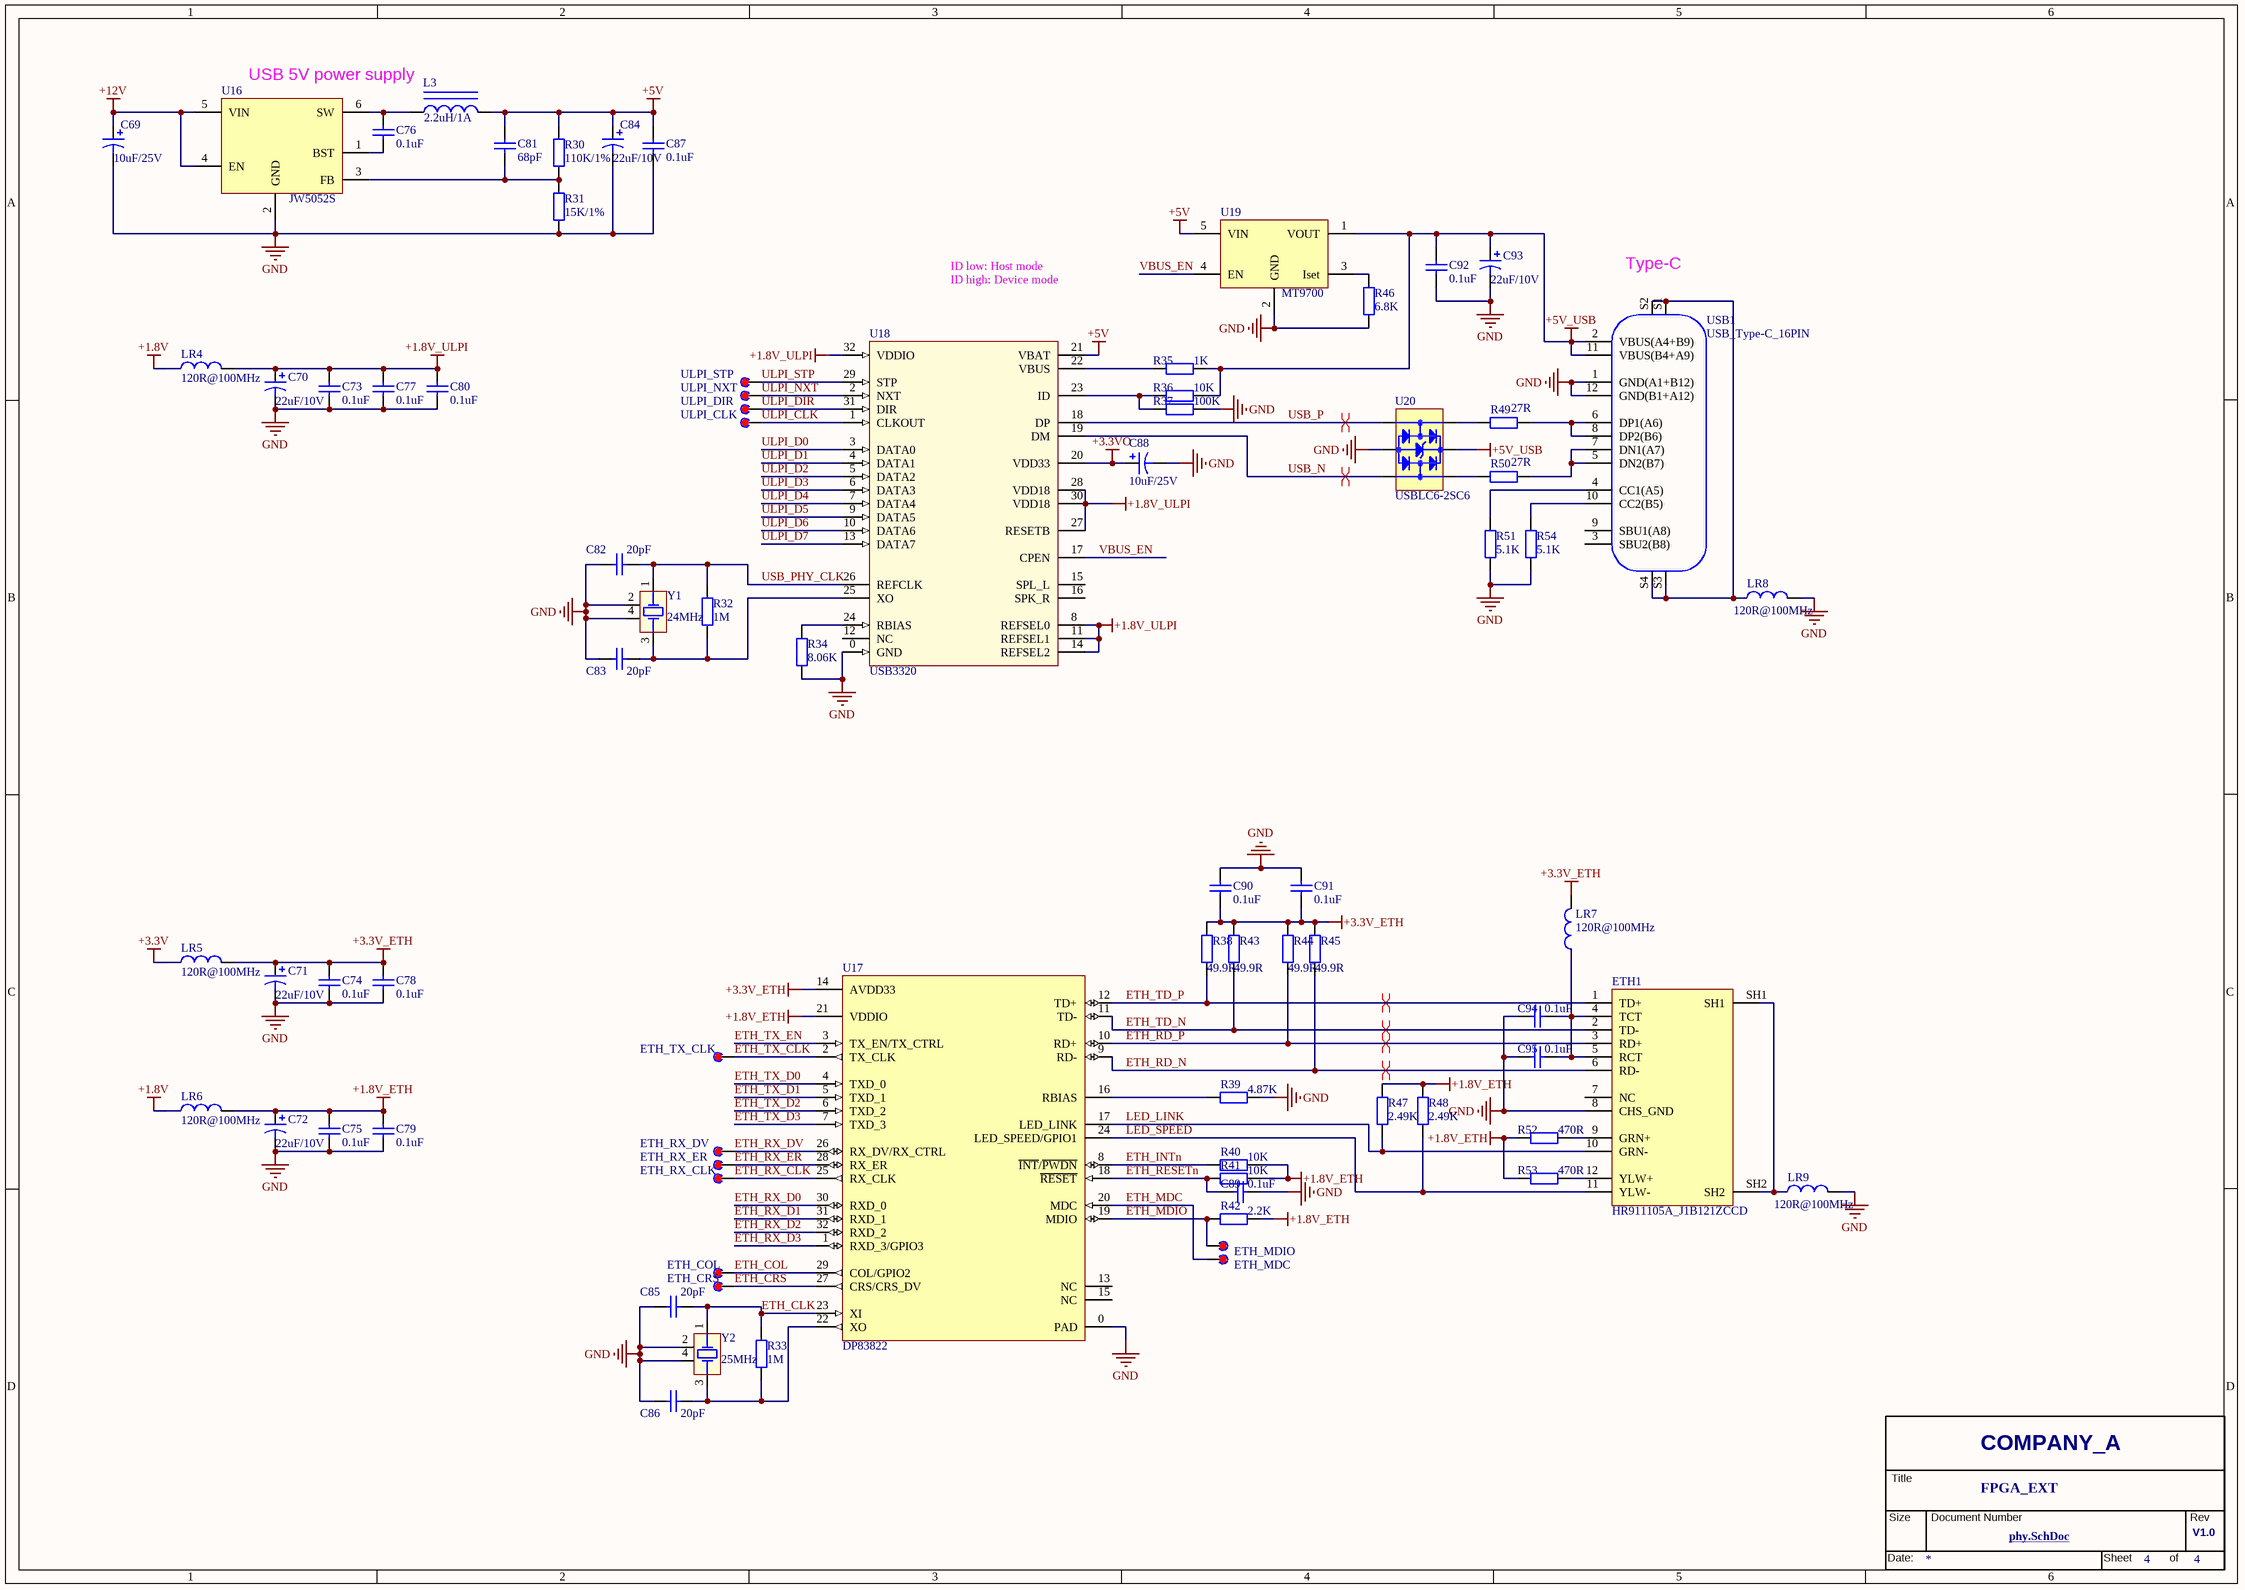
[diagram p0: MISC105414-8.SchDoc]
# Altium project MISC105414-4.PrjPcb (part 3 of 3)

## Sheet MISC105414-8.SchDoc
size 420 x 297 mm; DocumentNumber: MISC105414; SheetNumber: 4; SheetTotal: 4

### Parts
(Parts that share a designator on the sheet are numbered #1, #2 ... from top to bottom, then left to right.)
*?#4  Page Count: 4  OrgName: COMPANY_A  Title: FPGA_EXT  RevCode: V1.0  Doc: phy.SchDoc  (hidden comment: TitleBlock_YHSCH)  (graphical)
C69  10uF/25V  [0603C_N]
C70  22uF/10V  [0603C_N]
C71  22uF/10V  [0603C_N]
C72  22uF/10V  [0603C_N]
C73  0.1uF  [0603C_N]
C74  0.1uF  [0603C_N]
C75  0.1uF  [0603C_N]
C76  0.1uF  [0603C_N]
C77  0.1uF  [0603C_N]
C78  0.1uF  [0603C_N]
C79  0.1uF  [0603C_N]
C80  0.1uF  [0603C_N]
C81  68pF  [0603C_N]
C82  20pF  [0603C_N]
C83  20pF  [0603C_N]
C84  22uF/10V  [0603C_N]
C85  20pF  [0603C_N]
C86  20pF  [0603C_N]
C87  0.1uF  [0603C_N]
C88  10uF/25V  [0603C_N]
C89  0.1uF  [0603C_N]
C90  0.1uF  [0603C_N]
C91  0.1uF  [0603C_N]
C92  0.1uF  [0603C_N]
C93  22uF/10V  [0603C_N]
C94  0.1uF  [0603C_N]
C95  0.1uF  [0603C_N]
ETH1  HR911105A_J1B121ZCCD  [RJ45_HR911003A]
L3  2.2uH/1A  [LD-5.5mm]
LR4  120R@100MHz  [0603R_N]
LR5  120R@100MHz  [0603R_N]
LR6  120R@100MHz  [0603R_N]
LR7  120R@100MHz  [0603R_N]
LR8  120R@100MHz  [0603R_N]
LR9  120R@100MHz  [0603R_N]
R30  110K/1%  [0603R_N]
R31  15K/1%  [0603R_N]
R32  1M  [0603R_N]
R33  1M  [0603R_N]
R34  8.06K  [0603R_N]
R35  1K  [0603R_N]
R36  10K  [0603R_N]
R37  100K  [0603R_N]
R38  49.9R  [0603R_N]
R39  4.87K  [0603R_N]
R40  10K  [0603R_N]
R41  10K  [0603R_N]
R42  2.2K  [0603R_N]
R43  49.9R  [0603R_N]
R44  49.9R  [0603R_N]
R45  49.9R  [0603R_N]
R46  6.8K  [0603R_N]
R47  2.49K  [0603R_N]
R48  2.49K  [0603R_N]
R49  27R  [0603R_N]
R50  27R  [0603R_N]
R51  5.1K  [0603R_N]
R52  470R  [0603R_N]
R53  470R  [0603R_N]
R54  5.1K  [0603R_N]
TP40  ETH_TX_CLK  [FZ_TP-SMD-Mini]
TP41  ETH_RX_DV  [FZ_TP-SMD-Mini]
TP42  ETH_RX_ER  [FZ_TP-SMD-Mini]
TP43  ETH_RX_CLK  [FZ_TP-SMD-Mini]
TP44  ETH_COL  [FZ_TP-SMD-Mini]
TP45  ETH_CRS  [FZ_TP-SMD-Mini]
TP46  ULPI_STP  [FZ_TP-SMD-Mini]
TP47  ULPI_NXT  [FZ_TP-SMD-Mini]
TP48  ULPI_DIR  [FZ_TP-SMD-Mini]
TP49  ULPI_CLK  [FZ_TP-SMD-Mini]
TP50  ETH_MDIO  [FZ_TP-SMD-Mini]
TP51  ETH_MDC  [FZ_TP-SMD-Mini]
U16  JW5052S  [SOT-23-6]
U17  DP83822  [QFN32 5X5]
U18  USB3320  [QFN32 5x5]
U19  MT9700  [SOT-23-5]
U20  USBLC6-2SC6  [SOT-23-6]
USB1  USB_Type-C_16PIN  [USB_Type-C_16PIN]
Y1  24MHz  [XTAL_SMD3225]
Y2  25MHz  [XTAL_SMD3225]

### Nets
+1.8V: LR4.2 LR6.2
+1.8V_ETH: C72.1 C75.2 C79.2 LR6.1 R40.1 R41.1 R42.1 R47.1 R48.1 R52.1 R53.1 U17.21(VDDIO)
+1.8V_ULPI: C70.1 C73.2 C77.2 C80.1 LR4.1 U18.8(REFSEL0) U18.11(REFSEL1) U18.14(REFSEL2) U18.27(RESETB) U18.28(VDD18) U18.30(VDD18) U18.32(VDDIO)
+3.3V: LR5.2
+3.3V_ETH: C71.1 C74.2 C78.2 C90.2 C91.2 LR5.1 LR7.1 R38.2 R43.2 R44.2 R45.2 U17.14(AVDD33)
+3.3VO: C88.1 U18.20(VDD33)
+5V: C81.1 C84.1 C87.2 L3.2 R30.1 U18.21(VBAT) U19.5(VIN)
+5V_USB: C92.1 C93.1 R35.2 R36.2 U19.1(VOUT) U20.5(Vbus) USB1.2(VBUS(A4+B9)) USB1.11(VBUS(B4+A9))
+12V: C69.1 U16.4(EN) U16.5(VIN)
GND: C69.2 C70.2 C71.2 C72.2 C73.1 C74.1 C75.1 C77.1 C78.1 C79.1 C80.2 C82.2 C83.2 C84.2 C85.2 C86.2 C87.1 C88.2 C89.1 C90.1 C91.1 C92.2 C93.2 C94.1 C95.1 ETH1.8(CHS_GND) LR8.1 LR9.1 R31.2 R34.2 R37.2 R39.1 R46.1 R51.1 R54.1 U16.2(GND) U17.0(PAD) U18.0(GND) U19.2(GND) U20.2(GND) USB1.1(GND(A1+B12)) USB1.12(GND(B1+A12)) Y1.2 Y1.4 Y2.2 Y2.4
ETH_CLK: C85.1 R33.2 U17.23(XI) Y2.1(OSC1)
ETH_COL: TP44.1 U17.29(COL/GPIO2)
ETH_CRS: TP45.1 U17.27(CRS/CRS_DV)
ETH_INTn: R40.2 U17.8(~{INT}/~{PWDN})
ETH_MDC: TP51.1 U17.20(MDC)
ETH_MDIO: R42.2 TP50.1 U17.19(MDIO)
ETH_RD_N: ETH1.6(RD-) R45.1 U17.9(RD-)
ETH_RD_P: ETH1.3(RD+) R44.1 U17.10(RD+)
ETH_RESETn: C89.2 R41.2 U17.18(~{RESET})
ETH_RX_CLK: TP43.1 U17.25(RX_CLK)
ETH_RX_D0: U17.30(RXD_0)
ETH_RX_D1: U17.31(RXD_1)
ETH_RX_D2: U17.32(RXD_2)
ETH_RX_D3: U17.1(RXD_3/GPIO3)
ETH_RX_DV: TP41.1 U17.26(RX_DV/RX_CTRL)
ETH_RX_ER: TP42.1 U17.28(RX_ER)
ETH_TD_N: ETH1.2(TD-) R43.1 U17.11(TD-)
ETH_TD_P: ETH1.1(TD+) R38.1 U17.12(TD+)
ETH_TX_CLK: TP40.1 U17.2(TX_CLK)
ETH_TX_D0: U17.4(TXD_0)
ETH_TX_D1: U17.5(TXD_1)
ETH_TX_D2: U17.6(TXD_2)
ETH_TX_D3: U17.7(TXD_3)
ETH_TX_EN: U17.3(TX_EN/TX_CTRL)
LED_LINK: ETH1.10(GRN-) R47.2 U17.17(LED_LINK)
LED_SPEED: ETH1.11(YLW-) R48.2 U17.24(LED_SPEED/GPIO1)
ULPI_CLK: TP49.1 U18.1(CLKOUT)
ULPI_D0: U18.3(DATA0)
ULPI_D1: U18.4(DATA1)
ULPI_D2: U18.5(DATA2)
ULPI_D3: U18.6(DATA3)
ULPI_D4: U18.7(DATA4)
ULPI_D5: U18.9(DATA5)
ULPI_D6: U18.10(DATA6)
ULPI_D7: U18.13(DATA7)
ULPI_DIR: TP48.1 U18.31(DIR)
ULPI_NXT: TP47.1 U18.2(NXT)
ULPI_STP: TP46.1 U18.29(STP)
USB_N: U18.19(DM) U20.1(CH1)
USB_P: U18.18(DP) U20.3(CH2)
USB_PHY_CLK: C82.1 R32.2 U18.26(REFCLK) Y1.1(OSC1)
VBUS_EN: U18.17(CPEN) U19.4(EN)
NetC76_1: C76.1 U16.1(BST)
NetC76_2: C76.2 L3.1 U16.6(SW)
NetC81_2: C81.2 R30.2 R31.1 U16.3(FB)
NetC83_1: C83.1 R32.1 U18.25(XO) Y1.3(OSC2)
NetC86_1: C86.1 R33.1 U17.22(XO) Y2.3(OSC2)
NetC94_2: C94.2 C95.2 ETH1.4(TCT) ETH1.5(RCT) LR7.2
NetETH1_9: ETH1.9(GRN+) R52.2
NetETH1_12: ETH1.12(YLW+) R53.2
NetETH1_SH1: ETH1.SH1 ETH1.SH2 LR9.2
NetLR8_2: LR8.2 USB1.S1 USB1.S2 USB1.S3 USB1.S4
NetR34_1: R34.1 U18.24(RBIAS)
NetR35_1: R35.1 U18.22(VBUS)
NetR36_1: R36.1 R37.1 U18.23(ID)
NetR39_2: R39.2 U17.16(RBIAS)
NetR46_2: R46.2 U19.3(Iset)
NetR49_1: R49.1 U20.4(CH3)
NetR49_2: R49.2 USB1.6(DP1(A6)) USB1.8(DP2(B6))
NetR50_1: R50.1 U20.6(CH4)
NetR50_2: R50.2 USB1.5(DN2(B7)) USB1.7(DN1(A7))
NetR51_2: R51.2 USB1.4(CC1(A5))
NetR54_2: R54.2 USB1.10(CC2(B5))

Not connected (* = marked no-connect by the designer): ETH1 7(NC); U17 13(NC) 15(NC); U18 12(NC) 15(SPL_L) 16(SPK_R); USB1 3(SBU2(B8)) 9(SBU1(A8))

### Layout directives
differential pair: ETH_RD_N, ETH_RD_P, ETH_TD_N, ETH_TD_P, USB_N, USB_P

### Notes on the sheet
- USB 5V power supply
- ID low: Host mode
- ID high: Device mode
- (near USB1) Type-C

### Library data of the parts
*?#4 = TitleBlock_YHSCH: Cage Code: 1; Page Number: 4; Page Modify Date: *
C69-C72 C84 C88 C93 = Cap Pol1: Polarized Capacitor (Radial); Value: 1uF; Published: 8-Jun-2000; LatestRevisionDate: 17-Jul-2002; LatestRevisionNote: Re-released for DXP Platform.; PackageReference: RB7.6-15; Publisher: Altium Limited
C73-C81 C87 C89-C92 C94 C95 = Cap: Capacitor; Value: 100nF; Published: 8-Jun-2000; LatestRevisionDate: 17-Jul-2002; LatestRevisionNote: Re-released for DXP Platform.; PackageReference: RAD-0.3; Publisher: Altium Limited
C82 C83 C85 C86 = Cap: Capacitor; Value: 0.1uF; Published: 8-Jun-2000; LatestRevisionDate: 17-Jul-2002; LatestRevisionNote: Re-released for DXP Platform.; PackageReference: RAD-0.3; Publisher: Altium Limited
ETH1 = HR911105A
L3 = Inductor Iron: Magnetic-Core Inductor; Published: 24-Mar-1999; LatestRevisionDate: 17-Jul-2002; LatestRevisionNote: Re-released for DXP Platform.; PackageReference: AXIAL-0.9; PackageDescription: Axial Device, Thru-Hole; 2 Leads; 0.9 in Pin Spacing; Publisher: Altium Limited
LR4-LR9 = L
R30-R54 = Res2: Resistor; Value: 4.7K; Published: 8-Jun-2000; LatestRevisionDate: 17-Jul-2002; LatestRevisionNote: Re-released for DXP Platform.; PackageReference: AXIAL-0.4; Publisher: Altium Limited
TP40-TP51 = TP_SMD
U16 = MP2359_JW5052S_SY8113B
U17 = DP83822_Eth PHY 10_100M w1588 802.3az
U18 = USB3320: USB_HS ULPI PHY
U19 = LPW5209_MT9700: Power switch 3.3V/5V
Y1 Y2 = XTAL_2

## Nets that join several sheets
+1.8V: MISC105414-3 (J1.E39 J1.F40 J1.G39 J1.H40), MISC105414-2 (5 pins), MISC105414-7 (45 pins), MISC105414-8 (LR4.2 LR6.2)
+3.3V: MISC105414-3 (5 pins), MISC105414-2 (13 pins), MISC105414-8 (LR5.2)
+12V: MISC105414-3 (5 pins), MISC105414-8 (C69.1 U16.4 U16.5)
GND: MISC105414-3 (244 pins), MISC105414-2 (70 pins), MISC105414-7 (45 pins), MISC105414-8 (46 pins)
DVP_D0: MISC105414-3 (J1.F16), MISC105414-2 (J5.24 R24.2)
DVP_D1: MISC105414-3 (J1.E16), MISC105414-2 (J5.23 R23.2)
DVP_D2: MISC105414-3 (J1.E13), MISC105414-2 (J5.19)
DVP_D3: MISC105414-3 (J1.F14), MISC105414-2 (J5.21)
DVP_D4: MISC105414-3 (J1.E15), MISC105414-2 (J5.22)
DVP_D5: MISC105414-3 (J1.F13), MISC105414-2 (J5.20)
DVP_D6: MISC105414-3 (J1.E12), MISC105414-2 (J5.18)
DVP_D7: MISC105414-3 (J1.F10), MISC105414-2 (J5.16)
DVP_D8: MISC105414-3 (J1.E10), MISC105414-2 (J5.14)
DVP_D9: MISC105414-3 (J1.E9), MISC105414-2 (J5.12)
DVP_HSYNC: MISC105414-3 (J1.E7), MISC105414-2 (J5.9 TP12.1)
DVP_MCLK: MISC105414-3 (J1.F8), MISC105414-2 (J5.13 TP16.1)
DVP_PCLK: MISC105414-3 (J1.F11), MISC105414-2 (J5.17 TP17.1)
DVP_PWDN: MISC105414-3 (J1.F7), MISC105414-2 (J5.8 TP11.1)
DVP_RST: MISC105414-3 (J1.E3), MISC105414-2 (J5.6 TP15.1)
DVP_SCL: MISC105414-3 (J1.F5), MISC105414-2 (J5.5 R26.1 TP14.1)
DVP_SDA: MISC105414-3 (J1.F4), MISC105414-2 (J5.3 R27.1 TP13.1)
DVP_STROBE: MISC105414-3 (J1.E2), MISC105414-2 (J5.1)
DVP_VSYNC: MISC105414-3 (J1.E6), MISC105414-2 (J5.7 TP10.1)
ETH_CLK: MISC105414-3 (J1.A38), MISC105414-8 (C85.1 R33.2 U17.23 Y2.1)
ETH_COL: MISC105414-3 (J1.K38), MISC105414-8 (TP44.1 U17.29)
ETH_CRS: MISC105414-3 (J1.G37), MISC105414-8 (TP45.1 U17.27)
ETH_INTn: MISC105414-3 (J1.K31), MISC105414-8 (R40.2 U17.8)
ETH_MDC: MISC105414-3 (J1.H31), MISC105414-8 (TP51.1 U17.20)
ETH_MDIO: MISC105414-3 (J1.H32), MISC105414-8 (R42.2 TP50.1 U17.19)
ETH_RESETn: MISC105414-3 (J1.K32), MISC105414-8 (C89.2 R41.2 U17.18)
ETH_RX_CLK: MISC105414-3 (J1.H38), MISC105414-8 (TP43.1 U17.25)
ETH_RX_D0: MISC105414-3 (J1.J37), MISC105414-8 (U17.30)
ETH_RX_D1: MISC105414-3 (J1.J36), MISC105414-8 (U17.31)
ETH_RX_D2: MISC105414-3 (J1.H35), MISC105414-8 (U17.32)
ETH_RX_D3: MISC105414-3 (J1.H34), MISC105414-8 (U17.1)
ETH_RX_DV: MISC105414-3 (J1.H37), MISC105414-8 (TP41.1 U17.26)
ETH_RX_ER: MISC105414-3 (J1.G36), MISC105414-8 (TP42.1 U17.28)
ETH_TX_CLK: MISC105414-3 (J1.G34), MISC105414-8 (TP40.1 U17.2)
ETH_TX_D0: MISC105414-3 (J1.K35), MISC105414-8 (U17.4)
ETH_TX_D1: MISC105414-3 (J1.K34), MISC105414-8 (U17.5)
ETH_TX_D2: MISC105414-3 (J1.J34), MISC105414-8 (U17.6)
ETH_TX_D3: MISC105414-3 (J1.J33), MISC105414-8 (U17.7)
ETH_TX_EN: MISC105414-3 (J1.G33), MISC105414-8 (U17.3)
EXT_IO0: MISC105414-3 (J1.Y2), MISC105414-2 (JE1.3)
EXT_IO1: MISC105414-3 (J1.A2), MISC105414-2 (JE1.4)
EXT_IO2: MISC105414-3 (J1.Y3), MISC105414-2 (JE1.5)
EXT_IO3: MISC105414-3 (J1.A3), MISC105414-2 (JE1.6)
EXT_IO4: MISC105414-3 (J1.Z4), MISC105414-2 (JE1.7)
EXT_IO5: MISC105414-3 (J1.B4), MISC105414-2 (JE1.8)
EXT_IO6: MISC105414-3 (J1.Z5), MISC105414-2 (JE1.9)
EXT_IO7: MISC105414-3 (J1.B5), MISC105414-2 (JE1.10)
EXT_IO8: MISC105414-3 (J1.Y6), MISC105414-2 (JE1.11)
EXT_IO9: MISC105414-3 (J1.A6), MISC105414-2 (JE1.12)
EXT_IO10: MISC105414-3 (J1.Y7), MISC105414-2 (JE1.13)
EXT_IO11: MISC105414-3 (J1.A7), MISC105414-2 (JE1.14)
EXT_IO12: MISC105414-3 (J1.Z8), MISC105414-2 (JE1.15)
EXT_IO13: MISC105414-3 (J1.B8), MISC105414-2 (JE1.16)
EXT_IO14: MISC105414-3 (J1.Z9), MISC105414-2 (JE1.17)
EXT_IO15: MISC105414-3 (J1.B9), MISC105414-2 (JE1.18)
EXT_IO16: MISC105414-3 (J1.Y10), MISC105414-2 (JE1.23)
EXT_IO17: MISC105414-3 (J1.A10), MISC105414-2 (JE1.24)
EXT_IO18: MISC105414-3 (J1.Y11), MISC105414-2 (JE1.25)
EXT_IO19: MISC105414-3 (J1.A11), MISC105414-2 (JE1.26)
EXT_IO20: MISC105414-3 (J1.Z12), MISC105414-2 (JE1.27)
EXT_IO21: MISC105414-3 (J1.B12), MISC105414-2 (JE1.28)
EXT_IO22: MISC105414-3 (J1.Z13), MISC105414-2 (JE1.29)
EXT_IO23: MISC105414-3 (J1.B13), MISC105414-2 (JE1.30)
EXT_IO24: MISC105414-3 (J1.Y14), MISC105414-2 (JE1.31)
EXT_IO25: MISC105414-3 (J1.A14), MISC105414-2 (JE1.32)
EXT_IO26: MISC105414-3 (J1.Y15), MISC105414-2 (JE1.33)
EXT_IO27: MISC105414-3 (J1.A15), MISC105414-2 (JE1.34)
EXT_IO28: MISC105414-3 (J1.Z16), MISC105414-2 (JE1.35)
EXT_IO29: MISC105414-3 (J1.B16), MISC105414-2 (JE1.36)
EXT_IO30: MISC105414-3 (J1.Z17), MISC105414-2 (JE1.37)
EXT_IO31: MISC105414-3 (J1.B17), MISC105414-2 (JE1.38)
EXT_IO32: MISC105414-3 (J1.Y18), MISC105414-2 (JE2.3)
EXT_IO33: MISC105414-3 (J1.A18), MISC105414-2 (JE2.4)
EXT_IO34: MISC105414-3 (J1.Y19), MISC105414-2 (JE2.5)
EXT_IO35: MISC105414-3 (J1.A19), MISC105414-2 (JE2.6)
EXT_IO36: MISC105414-3 (J1.Z20), MISC105414-2 (JE2.7)
EXT_IO37: MISC105414-3 (J1.B20), MISC105414-2 (JE2.8)
EXT_IO38: MISC105414-3 (J1.Z21), MISC105414-2 (JE2.9)
EXT_IO39: MISC105414-3 (J1.B21), MISC105414-2 (JE2.10)
EXT_IO40: MISC105414-3 (J1.Y22), MISC105414-2 (JE2.11)
EXT_IO41: MISC105414-3 (J1.A22), MISC105414-2 (JE2.12)
EXT_IO42: MISC105414-3 (J1.Y23), MISC105414-2 (JE2.13)
EXT_IO43: MISC105414-3 (J1.A23), MISC105414-2 (JE2.14)
EXT_IO44: MISC105414-3 (J1.Z24), MISC105414-2 (JE2.15)
EXT_IO45: MISC105414-3 (J1.B24), MISC105414-2 (JE2.16)
EXT_IO46: MISC105414-3 (J1.Z25), MISC105414-2 (JE2.17)
EXT_IO47: MISC105414-3 (J1.B25), MISC105414-2 (JE2.18)
EXT_IO48: MISC105414-3 (J1.Y26), MISC105414-2 (JE2.23)
EXT_IO49: MISC105414-3 (J1.A26), MISC105414-2 (JE2.24)
EXT_IO50: MISC105414-3 (J1.Y27), MISC105414-2 (JE2.25)
EXT_IO51: MISC105414-3 (J1.A27), MISC105414-2 (JE2.26)
EXT_IO52: MISC105414-3 (J1.Z28), MISC105414-2 (JE2.27)
EXT_IO53: MISC105414-3 (J1.B28), MISC105414-2 (JE2.28)
EXT_IO54: MISC105414-3 (J1.Z29), MISC105414-2 (JE2.29)
EXT_IO55: MISC105414-3 (J1.B29), MISC105414-2 (JE2.30)
EXT_IO56: MISC105414-3 (J1.Y30), MISC105414-2 (JE2.31)
EXT_IO57: MISC105414-3 (J1.A30), MISC105414-2 (JE2.32)
EXT_IO58: MISC105414-3 (J1.Y31), MISC105414-2 (JE2.33)
EXT_IO59: MISC105414-3 (J1.A31), MISC105414-2 (JE2.34)
EXT_IO60: MISC105414-3 (J1.B32), MISC105414-2 (JE2.35)
EXT_IO61: MISC105414-3 (J1.B33), MISC105414-2 (JE2.36)
EXT_IO62: MISC105414-3 (J1.A34), MISC105414-2 (JE2.37)
EXT_IO63: MISC105414-3 (J1.A35), MISC105414-2 (JE2.38)
LCD_B0: MISC105414-3 (J1.D17), MISC105414-2 (J2.19 J3.21)
LCD_B1: MISC105414-3 (J1.D18), MISC105414-2 (J2.18 J3.22)
LCD_B2: MISC105414-3 (J1.C18), MISC105414-2 (J2.17 J3.23)
LCD_B3: MISC105414-3 (J1.C19), MISC105414-2 (J2.16 J3.24)
LCD_B4: MISC105414-3 (J1.D20), MISC105414-2 (J2.15 J3.25)
LCD_B5: MISC105414-3 (J1.D21), MISC105414-2 (J2.14 J3.26)
LCD_B6: MISC105414-3 (J1.C22), MISC105414-2 (J2.13 J3.27)
LCD_B7: MISC105414-3 (J1.C23), MISC105414-2 (J2.12 J3.28 R6.1 R7.2)
LCD_CLK: MISC105414-3 (J1.D23), MISC105414-2 (J2.37 J3.30 TP7.1)
LCD_DE: MISC105414-3 (J1.D26), MISC105414-2 (J2.9 J3.34 TP4.1)
LCD_DISP: MISC105414-3 (J1.D24), MISC105414-2 (J3.31)
LCD_G0: MISC105414-3 (J1.C10), MISC105414-2 (J2.27 J3.13)
LCD_G1: MISC105414-3 (J1.C11), MISC105414-2 (J2.26 J3.14)
LCD_G2: MISC105414-3 (J1.D11), MISC105414-2 (J2.25 J3.15)
LCD_G3: MISC105414-3 (J1.D12), MISC105414-2 (J2.24 J3.16)
LCD_G4: MISC105414-3 (J1.C14), MISC105414-2 (J2.23 J3.17)
LCD_G5: MISC105414-3 (J1.C15), MISC105414-2 (J2.22 J3.18)
LCD_G6: MISC105414-3 (J1.D14), MISC105414-2 (J2.21 J3.19)
LCD_G7: MISC105414-3 (J1.D15), MISC105414-2 (J2.20 J3.20 R3.1 R4.2)
LCD_HSYNC: MISC105414-3 (J1.C26), MISC105414-2 (J2.11 J3.32 TP6.1)
LCD_R0: MISC105414-3 (J1.C2), MISC105414-2 (J2.35 J3.5)
LCD_R1: MISC105414-3 (J1.C3), MISC105414-2 (J2.34 J3.6)
LCD_R2: MISC105414-3 (J1.D4), MISC105414-2 (J2.33 J3.7)
LCD_R3: MISC105414-3 (J1.D5), MISC105414-2 (J2.32 J3.8)
LCD_R4: MISC105414-3 (J1.C6), MISC105414-2 (J2.31 J3.9)
LCD_R5: MISC105414-3 (J1.C7), MISC105414-2 (J2.30 J3.10)
LCD_R6: MISC105414-3 (J1.D8), MISC105414-2 (J2.29 J3.11)
LCD_R7: MISC105414-3 (J1.D9), MISC105414-2 (J2.28 J3.12 R1.1 R2.2)
LCD_TP_INT: MISC105414-3 (J1.D27), MISC105414-2 (J4.4)
LCD_TP_SCL: MISC105414-3 (J1.C31), MISC105414-2 (J4.6 R18.1 TP8.1)
LCD_TP_SDA: MISC105414-3 (J1.C30), MISC105414-2 (J4.5 R17.1 TP9.1)
LCD_VSYNC: MISC105414-3 (J1.C27), MISC105414-2 (J2.10 J3.33 TP5.1)
NOR2_CS: MISC105414-3 (J1.M3), MISC105414-7 (TP21.1 U10.7)
NOR_CS: MISC105414-3 (J1.J6), MISC105414-7 (TP35.1 U13.7)
NOR_D0: MISC105414-3 (J1.K7), MISC105414-7 (RP12.2 U13.15)
NOR_D1: MISC105414-3 (J1.K8), MISC105414-7 (RP12.4 U13.8)
NOR_D2: MISC105414-3 (J1.J9), MISC105414-7 (RP12.1 U13.9)
NOR_D3: MISC105414-3 (J1.J10), MISC105414-7 (RP12.3 U13.1)
NOR_D4: MISC105414-3 (J1.K10), MISC105414-7 (U13.14)
NOR_D5: MISC105414-3 (J1.K11), MISC105414-7 (U13.5)
NOR_D6: MISC105414-3 (J1.J12), MISC105414-7 (U13.12)
NOR_D7: MISC105414-3 (J1.J13), MISC105414-7 (U13.4)
NOR_DQS: MISC105414-3 (J1.K13), MISC105414-7 (TP37.1 U13.13)
NOR_SCLK: MISC105414-3 (J1.J7), MISC105414-7 (R29.2 TP36.1 U13.16)
NORE_CS: MISC105414-3 (J1.K14), MISC105414-7 (TP39.1 U15.1)
PS_CS: MISC105414-3 (J1.L4), MISC105414-7 (TP18.1 U9.A3)
PS_D0: MISC105414-3 (J1.M6), MISC105414-7 (RP11.3 U9.D3 U10.15)
PS_D1: MISC105414-3 (J1.M7), MISC105414-7 (RP11.4 U9.D2 U10.8)
PS_D2: MISC105414-3 (J1.L8), MISC105414-7 (RP11.1 U9.C4 U10.9)
PS_D3: MISC105414-3 (J1.L9), MISC105414-7 (RP11.2 U9.D4 U10.1)
PS_D4: MISC105414-3 (J1.L12), MISC105414-7 (U9.D5 U10.14)
PS_D5: MISC105414-3 (J1.L13), MISC105414-7 (U9.E3 U10.5)
PS_D6: MISC105414-3 (J1.M10), MISC105414-7 (U9.E2 U10.12)
PS_D7: MISC105414-3 (J1.M11), MISC105414-7 (U9.E1 U10.4)
PS_DQS: MISC105414-3 (J1.M14), MISC105414-7 (TP20.1 U9.C3 U10.13)
PS_RSTn: MISC105414-3 (J1.M15), MISC105414-7 (U9.A4 U10.3)
PS_SCLK: MISC105414-3 (J1.L5), MISC105414-7 (R28.2 TP19.1 U9.B2 U10.16)
PSE_CS: MISC105414-3 (J1.M2), MISC105414-7 (TP34.1 U12.1)
SDR_A0: MISC105414-3 (J1.K19), MISC105414-7 (U11.G8)
SDR_A1: MISC105414-3 (J1.K20), MISC105414-7 (U11.G9)
SDR_A2: MISC105414-3 (J1.J24), MISC105414-7 (U11.F7)
SDR_A3: MISC105414-3 (J1.J25), MISC105414-7 (U11.F3)
SDR_A4: MISC105414-3 (J1.K22), MISC105414-7 (U11.G1)
SDR_A5: MISC105414-3 (J1.K23), MISC105414-7 (U11.G2)
SDR_A6: MISC105414-3 (J1.J27), MISC105414-7 (U11.G3)
SDR_A7: MISC105414-3 (J1.J28), MISC105414-7 (U11.H1)
SDR_A8: MISC105414-3 (J1.K25), MISC105414-7 (U11.H2)
SDR_A9: MISC105414-3 (J1.K26), MISC105414-7 (U11.J3)
SDR_A10: MISC105414-3 (J1.J30), MISC105414-7 (U11.G7)
SDR_A11: MISC105414-3 (J1.J31), MISC105414-7 (U11.H9)
SDR_A12: MISC105414-3 (J1.G6), MISC105414-7 (U11.H3)
SDR_A13: MISC105414-3 (J1.G7), MISC105414-7 (U11.H7)
SDR_BA0: MISC105414-3 (J1.K28), MISC105414-7 (TP22.1 U11.J7)
SDR_BA1: MISC105414-3 (J1.K29), MISC105414-7 (TP23.1 U11.H8)
SDR_CAS: MISC105414-3 (J1.H17), MISC105414-7 (TP25.1 U11.K7)
SDR_CKE: MISC105414-3 (J1.H14), MISC105414-7 (TP33.1 U11.J2)
SDR_CLK: MISC105414-3 (J1.H13), MISC105414-7 (TP32.1 U11.J1)
SDR_CS: MISC105414-3 (J1.G16), MISC105414-7 (TP27.1 U11.J8)
SDR_D0: MISC105414-3 (J1.H22), MISC105414-7 (U11.R8)
SDR_D1: MISC105414-3 (J1.H23), MISC105414-7 (U11.N7)
SDR_D2: MISC105414-3 (J1.G24), MISC105414-7 (U11.R9)
SDR_D3: MISC105414-3 (J1.G25), MISC105414-7 (U11.N8)
SDR_D4: MISC105414-3 (J1.H25), MISC105414-7 (U11.P9)
SDR_D5: MISC105414-3 (J1.H26), MISC105414-7 (U11.M8)
SDR_D6: MISC105414-3 (J1.G27), MISC105414-7 (U11.M7)
SDR_D7: MISC105414-3 (J1.G28), MISC105414-7 (U11.L8)
SDR_D8: MISC105414-3 (J1.H28), MISC105414-7 (U11.L2)
SDR_D9: MISC105414-3 (J1.H29), MISC105414-7 (U11.M3)
SDR_D10: MISC105414-3 (J1.G30), MISC105414-7 (U11.M2)
SDR_D11: MISC105414-3 (J1.G31), MISC105414-7 (U11.P1)
SDR_D12: MISC105414-3 (J1.M18), MISC105414-7 (U11.N2)
SDR_D13: MISC105414-3 (J1.M19), MISC105414-7 (U11.R1)
SDR_D14: MISC105414-3 (J1.L16), MISC105414-7 (U11.N3)
SDR_D15: MISC105414-3 (J1.L17), MISC105414-7 (U11.R2)
SDR_D16: MISC105414-3 (J1.M22), MISC105414-7 (U11.E8)
SDR_D17: MISC105414-3 (J1.M23), MISC105414-7 (U11.D7)
SDR_D18: MISC105414-3 (J1.L20), MISC105414-7 (U11.D8)
SDR_D19: MISC105414-3 (J1.L21), MISC105414-7 (U11.B9)
SDR_D20: MISC105414-3 (J1.J18), MISC105414-7 (U11.C8)
SDR_D21: MISC105414-3 (J1.J19), MISC105414-7 (U11.A9)
SDR_D22: MISC105414-3 (J1.L24), MISC105414-7 (U11.C7)
SDR_D23: MISC105414-3 (J1.L25), MISC105414-7 (U11.A8)
SDR_D24: MISC105414-3 (J1.G22), MISC105414-7 (U11.A2)
SDR_D25: MISC105414-3 (J1.L29), MISC105414-7 (U11.C3)
SDR_D26: MISC105414-3 (J1.G21), MISC105414-7 (U11.A1)
SDR_D27: MISC105414-3 (J1.L28), MISC105414-7 (U11.C2)
SDR_D28: MISC105414-3 (J1.K16), MISC105414-7 (U11.B1)
SDR_D29: MISC105414-3 (J1.K17), MISC105414-7 (U11.D2)
SDR_D30: MISC105414-3 (J1.J21), MISC105414-7 (U11.D3)
SDR_D31: MISC105414-3 (J1.J22), MISC105414-7 (U11.E2)
SDR_DQM0: MISC105414-3 (J1.G18), MISC105414-7 (TP28.1 U11.K9)
SDR_DQM1: MISC105414-3 (J1.G19), MISC105414-7 (TP29.1 U11.K1)
SDR_DQM2: MISC105414-3 (J1.H19), MISC105414-7 (TP30.1 U11.F8)
SDR_DQM3: MISC105414-3 (J1.H20), MISC105414-7 (TP31.1 U11.F2)
SDR_RAS: MISC105414-3 (J1.H16), MISC105414-7 (TP24.1 U11.J9)
SDR_WE: MISC105414-3 (J1.G15), MISC105414-7 (TP26.1 U11.K8)
ULPI_CLK: MISC105414-3 (J1.E37), MISC105414-8 (TP49.1 U18.1)
ULPI_D0: MISC105414-3 (J1.F35), MISC105414-8 (U18.3)
ULPI_D1: MISC105414-3 (J1.F34), MISC105414-8 (U18.4)
ULPI_D2: MISC105414-3 (J1.E34), MISC105414-8 (U18.5)
ULPI_D3: MISC105414-3 (J1.E33), MISC105414-8 (U18.6)
ULPI_D4: MISC105414-3 (J1.D33), MISC105414-8 (U18.7)
ULPI_D5: MISC105414-3 (J1.D31), MISC105414-8 (U18.9)
ULPI_D6: MISC105414-3 (J1.D30), MISC105414-8 (U18.10)
ULPI_D7: MISC105414-3 (J1.D29), MISC105414-8 (U18.13)
ULPI_DIR: MISC105414-3 (J1.F37), MISC105414-8 (TP48.1 U18.31)
ULPI_NXT: MISC105414-3 (J1.E36), MISC105414-8 (TP47.1 U18.2)
ULPI_STP: MISC105414-3 (J1.F38), MISC105414-8 (TP46.1 U18.29)
USB_PHY_CLK: MISC105414-3 (J1.A39), MISC105414-8 (C82.1 R32.2 U18.26 Y1.1)